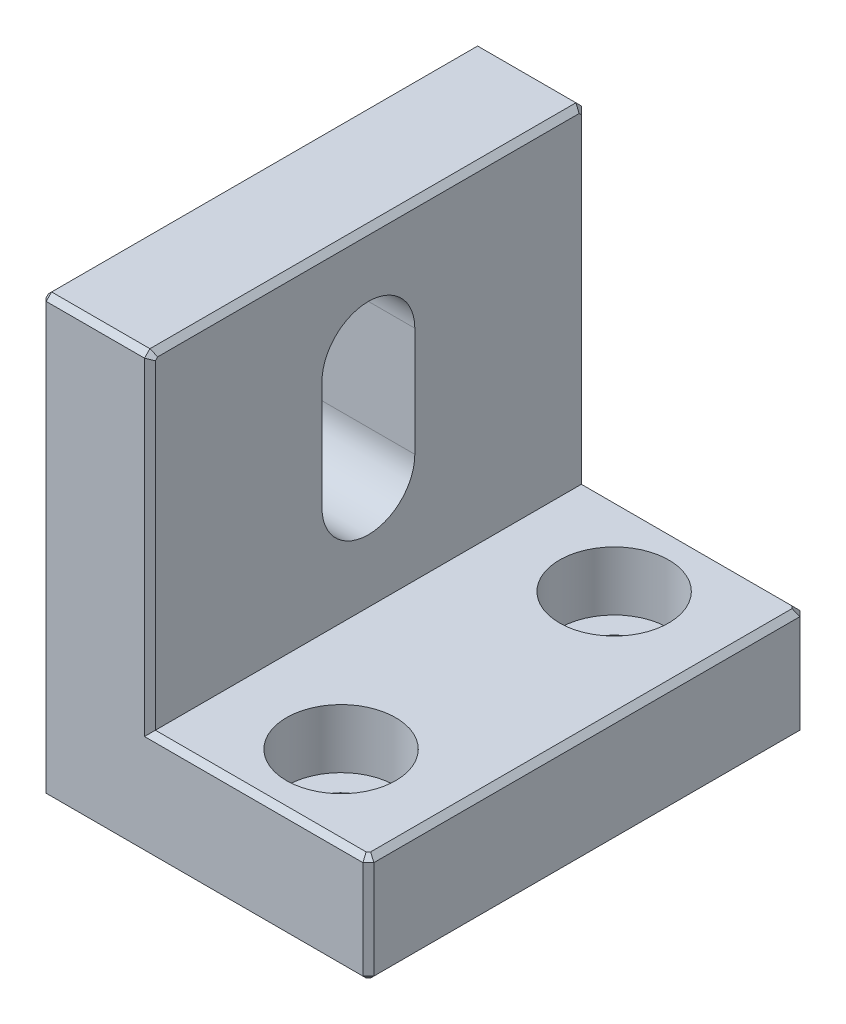
SolidWorks part; units mm, degrees
ref_plane "Front" through (0, 0, 0) normal (0, 0, 1) x (1, 0, 0)
ref_plane "Top" through (0, 0, 0) normal (0, 1, 0) x (1, 0, 0)
ref_plane "Right" through (0, 0, 0) normal (1, 0, 0) x (0, 0, -1)
sketch "草图1" plane through (0, 0, 0) normal (0, 1, 0) x (1, 0, 0)
  line L1 (-15, 20) -> (15, 20)
  line L2 (-15, 20) -> (-15, -20)
  line L3 (-15, -20) -> (15, -20)
  line L4 (15, 20) -> (15, -20)
  line L5 (-15, 20) -> (15, -20) construction
  line L6 (-15, -20) -> (15, 20) construction
  point P0 (0, 0)
  dimension "D1" = 30
  dimension "D2" = 40
extrude "凸台-拉伸1" add sketch "草图1" along normal blind 10
sketch "草图2" plane through (-15, 0, 0) normal (-1, 0, 0) x (0, 0, 1)
  line L0 (20, 10) -> (20, 0) construction
  line L1 (-20, 0) -> (20, 0)
  line L2 (-20, 0) -> (-20, 40)
  line L3 (-20, 40) -> (20, 40)
  line L4 (20, 0) -> (20, 40)
  dimension "D1" = 40
extrude "凸台-拉伸2" add sketch "草图2" against normal blind 10
hole_wizard "M5 六角凹头螺钉的柱形沉头孔1" positions "草图4" profile "草图3" counterbore size "M5" standard "Iso" end condition through all
sketch "草图4" plane through (0, 10, 0) normal (0, 1, 0) x (1, 0, 0)
  line L0 (-5, 0) -> (15, 0) construction
  line L1 (-5, -20) -> (-5, 20) construction
  line L2 (15, -20) -> (15, 20) construction
  point P0 (5, -12.5)
  point P2 (5, 12.5)
  dimension "D1" = 25
  dimension "D2" = 10
sketch "草图3" plane through (5, 10, 12.5) normal (1, 0, 0) x (0, 0, 1)
  line L0 (0, 0) -> (0, 10)
  line L1 (0, 10) -> (2.75, 10)
  line L3 (2.75, 10) -> (2.75, 5.4)
  line L4 (2.75, 5.4) -> (5, 5.4)
  line L5 (5, 5.4) -> (5, 0)
  line L7 (5, 0) -> (0, 0)
  line L11 (0, -6.35) -> (0, 107.95) construction
  dimension "通孔孔直径" = 5.5
  dimension "通孔孔深度" = 10
  dimension "柱形沉头孔直径" = 10
  dimension "柱形沉头孔深度" = 5.4
chamfer "倒角1" distance 0.5 angle 45 2 edges at (15, 5, -20) (15, 5, 20)
sketch "草图5" plane through (-5, 0, 0) normal (1, 0, 0) x (0, 0, -1)
  line L0 (0, 40) -> (0, 10) construction
  line L1 (-20, 40) -> (20, 40) construction
  line L2 (-19.5, 10) -> (19.5, 10) construction
  line L3 (0, 30) -> (0, 20) construction
  line L4 (4.25, 30) -> (4.25, 20)
  line L5 (-4.25, 30) -> (-4.25, 20)
  arc A0 (4.25, 30) -> (-4.25, 30) centre (0, 30) ccw
  arc A1 (-4.25, 20) -> (4.25, 20) centre (0, 20) ccw
  point P8 (0, 25)
  dimension "D1" = 8.5
  dimension "D2" = 10
  dimension "D3" = 10
extrude "切除-拉伸1" cut sketch "草图5" against normal through all
chamfer "倒角2" distance 0.5 angle 45 2 edges at (-10, 40, 20) (-10, 40, -20)
chamfer "倒角3" distance 0.5 angle 45 21 edges at (-15, 19.75, 20) (-15, 39.75, 19.75) (-15, 40, 0) (-5, 40, 0) (-15, 39.75, -19.75) (-15, 19.75, -20) (-15, 0, 0) (-0.25, 0, -20) (14.75, 0, -19.75) (-0.25, 0, 20) (14.75, 0, 19.75) (15, 0, 0) (14.75, 10, 19.75) (4.75, 10, 20) (-5, 24.75, 20) (-5, 39.75, 19.75) (-5, 39.75, -19.75) (-5, 24.75, -20) (4.75, 10, -20) (14.75, 10, -19.75) (15, 10, 0)
